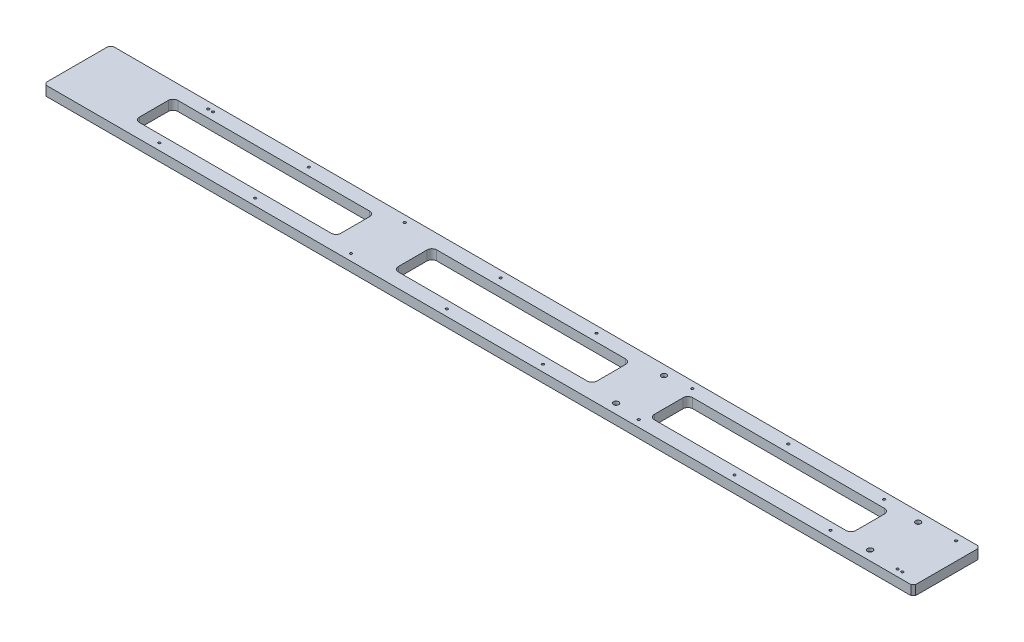
from build123d import *

# Parameters (mm, degrees)
SKETCH_1_W                   = 1814
SKETCH_1_H                   = 140
EXTRUDE_1_DEPTH              = 20
CHAMFER_1_SIZE               = 5
HOLE_WIZARD_M6_1_D           = 6.6
HOLE_WIZARD_M6_1_CBORE_D     = 11
HOLE_WIZARD_M6_1_CBORE_DEPTH = 6.8
SKETCH_5_W                   = 420
SKETCH_5_H                   = 80
SKETCH_5_W_2                 = 414
CUT_EXTRUDE_1_DEPTH          = 910.917029185
FILLET_2_R                   = 10
HOLE_WIZARD_M6_1_2_D         = 5
F_5_0MM_1_D                  = 5
F_5_0MM_1_DEPTH              = 15
F_5_0MM_1_TIP                = 1.502151548


with BuildPart() as part:
    # 草图1 → 凸台-拉伸1 (new body)
    with BuildSketch(Plane(origin=(0, 0, 0), x_dir=(1, 0, 0), z_dir=(0, 1, 0))):
        Rectangle(SKETCH_1_W, SKETCH_1_H)
    extrude(amount=EXTRUDE_1_DEPTH)

    # 倒角1
    chamfer_1_edges = [part.edges().sort_by_distance(p)[0] for p in [
        (907, 10, 70),
        (-907, 10, 70),
        (-907, 10, -70),
        (907, 10, -70),
    ]]
    chamfer(chamfer_1_edges, length=CHAMFER_1_SIZE)

    # Hole Wizard M6 _1 (through all)
    with Locations(Plane(origin=(0, 20, 0), x_dir=(1, 0, 0), z_dir=(0, 1, 0))):
        with Locations((267, 50), (797, 50), (797, -50), (267, -50)):
            CounterBoreHole(HOLE_WIZARD_M6_1_D / 2, HOLE_WIZARD_M6_1_CBORE_D / 2, HOLE_WIZARD_M6_1_CBORE_DEPTH)

    # 草图5 → 切除-拉伸1 (cut, through all)
    with BuildSketch(Plane.XZ):
        with Locations((537, 0)):
            Rectangle(SKETCH_5_W, SKETCH_5_H)
        Rectangle(SKETCH_5_W_2, SKETCH_5_H)
        with Locations((-537, 0)):
            Rectangle(SKETCH_5_W, SKETCH_5_H)
    extrude(amount=-CUT_EXTRUDE_1_DEPTH, mode=Mode.SUBTRACT)

    # 圆角2
    fillet_2_edges = [part.edges().sort_by_distance(p)[0] for p in [
        (-747, 10, 40),
        (-327, 10, 40),
        (-327, 10, -40),
        (-747, 10, -40),
        (327, 10, -40),
        (327, 10, 40),
        (747, 10, 40),
        (747, 10, -40),
        (-207, 10, -40),
        (-207, 10, 40),
        (207, 10, 40),
        (207, 10, -40),
    ]]
    fillet(fillet_2_edges, radius=FILLET_2_R)

    # Hole Wizard M6 _1 2 (through all)
    with Locations(Plane(origin=(0, 20, 0), x_dir=(1, 0, 0), z_dir=(0, 1, 0))):
        with Locations((-679.749998444, 56), (-479.749998444, 56), (-279.749998444, 56), (-79.749998444, 56), (120.250001556, 56), (320.250001556, 56), (520.250001556, 56), (720.250001556, 56), (870.250001556, 56), (870.250001556, -56), (720.250001556, -56), (520.250001556, -56), (320.250001556, -56), (120.250001556, -56), (-79.749998444, -56), (-279.749998444, -56), (-479.749998444, -56), (-679.749998444, -56)):
            Hole(HOLE_WIZARD_M6_1_2_D / 2)

    # Ø5.0mm 暗销孔1
    with Locations(Plane(origin=(0, 20, 0), x_dir=(1, 0, 0), z_dir=(0, 1, 0))):
        with Locations((-689.749998444, 56), (860.250001556, -56)):
            Hole(F_5_0MM_1_D / 2, depth=F_5_0MM_1_DEPTH)
            with Locations((0, 0, -(F_5_0MM_1_DEPTH + F_5_0MM_1_TIP / 2))):  # 118° drill point
                Cone(0, F_5_0MM_1_D / 2, F_5_0MM_1_TIP, mode=Mode.SUBTRACT)


solid = part.part
